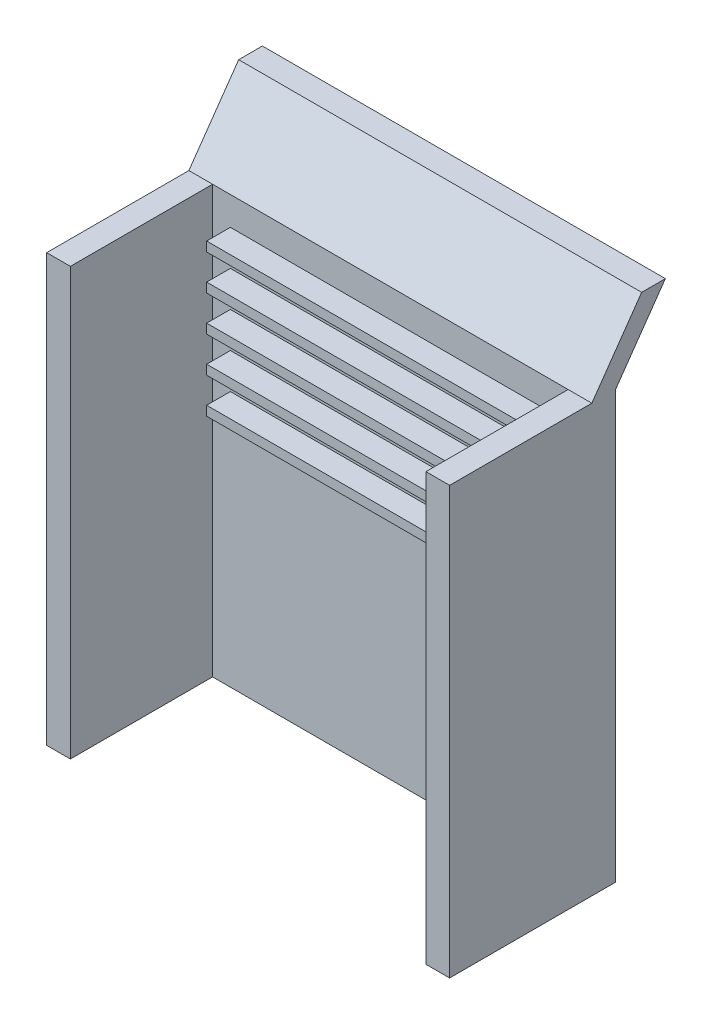
from build123d import *

# Parameters (mm, degrees)
SKETCH_1_W             = 170
SKETCH_1_H             = 180
EXTRUDE_1_DEPTH        = 10
SKETCH_2_W             = 10
SKETCH_2_H             = 180
EXTRUDE_2_DEPTH        = 60
EXTRUDE_3_REACH        = 206.695
SKETCH_4_W             = 135
SKETCH_4_H             = 4
EXTRUDE_4_DEPTH        = 10
PATTERN_LINEAR_1_COUNT = 5
PATTERN_LINEAR_1_PITCH = 15


with BuildPart() as part:
    # 草图1 → 凸台-拉伸1 (new body)
    with BuildSketch(Plane.XY):
        Rectangle(SKETCH_1_W, SKETCH_1_H)
    extrude(amount=EXTRUDE_1_DEPTH)

    # 草图2 → 凸台-拉伸2 (add)
    with BuildSketch(Plane.XY.offset(10)):
        with Locations((-80, 0)):
            Rectangle(SKETCH_2_W, SKETCH_2_H)
        with Locations((80, 0)):
            Rectangle(SKETCH_2_W, SKETCH_2_H)
    extrude(amount=EXTRUDE_2_DEPTH)

    # 凸台-拉伸3: up to this face of the body (flat: up to its plane)
    extrude_3_end = Plane(part.part.faces().sort_by_distance((-85, 0, 35))[0])
    # 草图3 → 凸台-拉伸3 (add, up to the picked face)
    with BuildSketch(Plane(origin=(85, 0, 0), x_dir=(0, 0, -1), z_dir=(1, 0, 0)), mode=Mode.PRIVATE) as extrude_3_sk1:
        Polygon((0, 90), (21.006226146, 120), (11.006226146, 120), (-10, 90), align=None)
    extrude_3_tool1 = split(extrude(extrude_3_sk1.sketch, amount=-EXTRUDE_3_REACH, mode=Mode.PRIVATE), bisect_by=extrude_3_end, keep=Keep.BOTH, mode=Mode.PRIVATE)
    add(extrude_3_tool1.solids().sort_by(Axis((85, 105, -5.503113), (-1, 0, 0)))[0])

    # 草图4 → 凸台-拉伸4 (add)
    with BuildSketch(Plane.XY.offset(10)):
        with Locations((0, 76)):
            Rectangle(SKETCH_4_W, SKETCH_4_H)
    extrude_4 = extrude(amount=EXTRUDE_4_DEPTH)

    # 阵列(线性)1: 凸台-拉伸4 ×5
    with Locations(*[(0, -i * PATTERN_LINEAR_1_PITCH, 0) for i in range(1, PATTERN_LINEAR_1_COUNT)]):
        add(extrude_4)


solid = part.part
